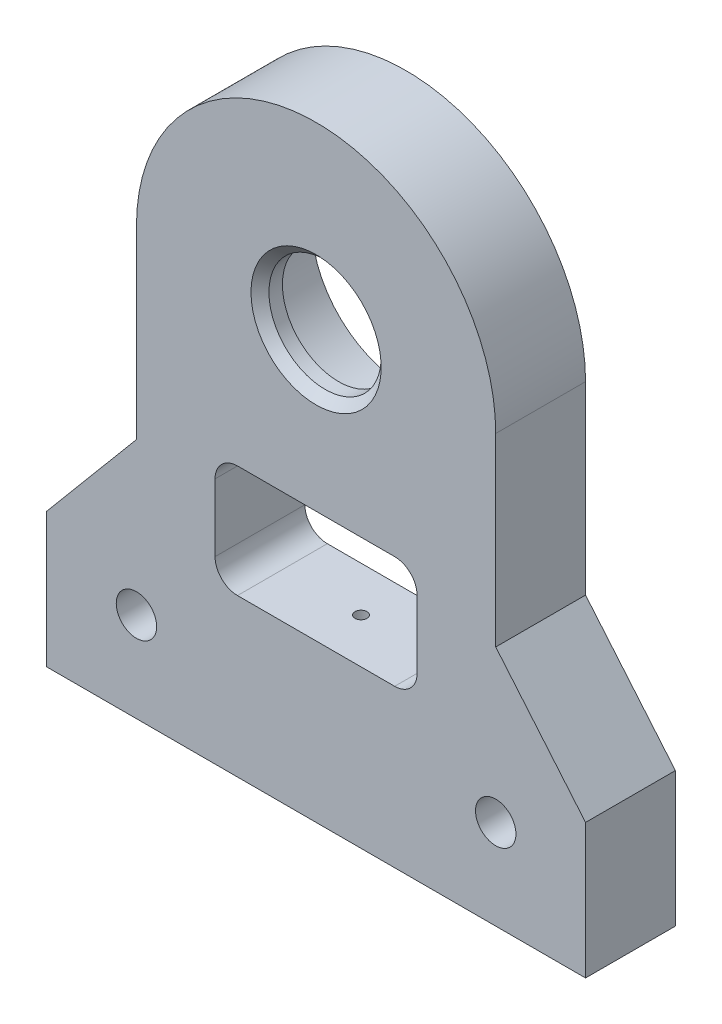
SolidWorks part; units mm, degrees
material "AL6061"
ref_plane "前视基准面" through (0, 0, 0) normal (0, 0, 1) x (1, 0, 0)
ref_plane "上视基准面" through (0, 0, 0) normal (0, 1, 0) x (1, 0, 0)
ref_plane "右视基准面" through (0, 0, 0) normal (1, 0, 0) x (0, 0, -1)
sketch "草图1" plane through (0, 0, 0) normal (0, 0, 1) x (1, 0, 0)
  line L0 (0, 73.4037) -> (0, -11.9326) construction
  line L1 (-60, 30) -> (-40, 53.8351)
  line L3 (-60, 30) -> (-60, 0)
  line L4 (-60, 0) -> (60, 0)
  line L5 (60, 30) -> (60, 0)
  line L6 (-40, 53.8351) -> (-40, 95)
  line L7 (60, 30) -> (40, 53.8351)
  line L8 (40, 53.8351) -> (40, 95)
  circle A1 centre (0, 95) radius 12.5
  arc A3 (-40, 95) -> (40, 95) centre (0, 95) cw
  dimension "D2" = 95
  dimension "D3" = 25
  dimension "D1" = 120
  dimension "D4" = 30
  dimension "D5" = 80
  dimension "D6" = 40
extrude "凸台-拉伸1" add sketch "草图1" along normal mid plane 20
hole_wizard "M8 螺纹孔1" positions "草图2" profile "草图3" tap size "M8" standard "GB"
sketch "草图2" plane through (0, 0, 0) normal (0, -1, 0) x (-1, 0, 0)
  line L0 (-54.3854, 0) -> (55.5026, 0) construction
  line L1 (0, 11.8825) -> (0, -11.8825) construction
  point P0 (50, 0)
  point P2 (0, 0)
  point P11 (-50, 0)
  dimension "D1" = 100
sketch "草图3" plane through (-50, 0, 0) normal (1, 0, 0) x (0, 0, -1)
  line L0 (0, 0) -> (0, 35.7929)
  line L1 (0, 35.7929) -> (3.4, 33.75)
  line L2 (3.4, 33.75) -> (3.4, 0)
  line L5 (3.4, 0) -> (0, 0)
  line L10 (0, 35.7929) -> (-3.4, 33.75) construction
  line L11 (0, -6.35) -> (0, 107.95) construction
  dimension "螺纹孔钻头直径" = 6.8
  dimension "螺纹孔钻头深度" = 33.75
  dimension "导头角度" = 118
cosmetic thread "孔螺蚊线1" parameters "D1"=30, "D2"=8
cosmetic thread "孔螺蚊线2" parameters "D1"=30, "D2"=8
cosmetic thread "孔螺蚊线3" parameters "D1"=30, "D2"=8
hole_wizard "Ø6.0 (6) 直径孔1" positions "草图4" profile "草图5" hole size "Ø6.0" standard "GB"
sketch "草图4" plane through (0, 0, 0) normal (0, -1, 0) x (-1, 0, 0)
  line L0 (-56.8228, 0) -> (54.8932, 0) construction
  line L1 (0, 11.3747) -> (0, -12.7966) construction
  point P0 (-35, 0)
  point P10 (35, 0)
  dimension "D1" = 70
sketch "草图5" plane through (35, 0, 0) normal (1, 0, 0) x (0, 0, -1)
  line L0 (0, 0) -> (0, 16.8026)
  line L1 (0, 16.8026) -> (3, 15)
  line L2 (3, 15) -> (3, 0)
  line L5 (3, 0) -> (0, 0)
  line L10 (0, 16.8026) -> (-3, 15) construction
  line L11 (0, -6.35) -> (0, 107.95) construction
  dimension "孔直径" = 6
  dimension "孔深度" = 15
  dimension "导头角度" = 118
sketch "草图6" plane through (0, 0, -10) normal (0, 0, 1) x (1, 0, 0)
  circle A0 centre (0, 95) radius 21
  dimension "D1" = 42
extrude "切除-拉伸1" cut sketch "草图6" along normal blind 15
chamfer "倒角1" distance 2 angle 45 1 edges at (12.5, 95, 10)
hole_wizard "打孔尺寸(%根据)内六角圆柱头螺钉的类型2" positions "草图11" profile "草图12" counterbore size "M8" standard "GB" end condition through all
sketch "草图11" plane through (0, 0, -10) normal (0, 0, -1) x (-1, 0, 0)
  line L0 (0, 150) -> (0, -8.5412) construction
  line L1 (60, 0) -> (-60, 0) construction
  point P0 (-40, 20)
  point P8 (40, 20)
  dimension "D1" = 80
  dimension "D2" = 20
sketch "草图12" plane through (40, 20, -10) normal (1, 0, 0) x (0, 1, 0)
  line L0 (0, 0) -> (0, 20)
  line L1 (0, 20) -> (4.5, 20)
  line L3 (4.5, 20) -> (4.5, 9)
  line L4 (4.5, 9) -> (7.5, 9)
  line L5 (7.5, 9) -> (7.5, 0)
  line L7 (7.5, 0) -> (0, 0)
  line L11 (0, -6.35) -> (0, 107.95) construction
  dimension "通孔孔直径" = 9
  dimension "通孔孔深度" = 20
  dimension "柱形沉头孔直径" = 15
  dimension "柱形沉头孔深度" = 9
sketch "草图13" plane through (0, 0, -10) normal (0, 0, -1) x (-1, 0, 0)
  line L0 (0, 151.4005) -> (0, -8.7458) construction
  line L1 (60, 0) -> (-60, 0) construction
  line L2 (17.5, 60) -> (-17.5, 60)
  line L3 (22.5, 55) -> (22.5, 40)
  line L4 (17.5, 35) -> (-17.5, 35)
  line L5 (-22.5, 55) -> (-22.5, 40)
  arc A0 (-17.5, 60) -> (-22.5, 55) centre (-17.5, 55) ccw
  arc A1 (22.5, 40) -> (17.5, 35) centre (17.5, 40) cw
  arc A2 (-17.5, 35) -> (-22.5, 40) centre (-17.5, 40) cw
  arc A3 (17.5, 60) -> (22.5, 55) centre (17.5, 55) cw
  dimension "D1" = 5
  dimension "D2" = 35
  dimension "D3" = 25
  dimension "D4" = 45
extrude "切除-拉伸2" cut sketch "草图13" against normal through all
